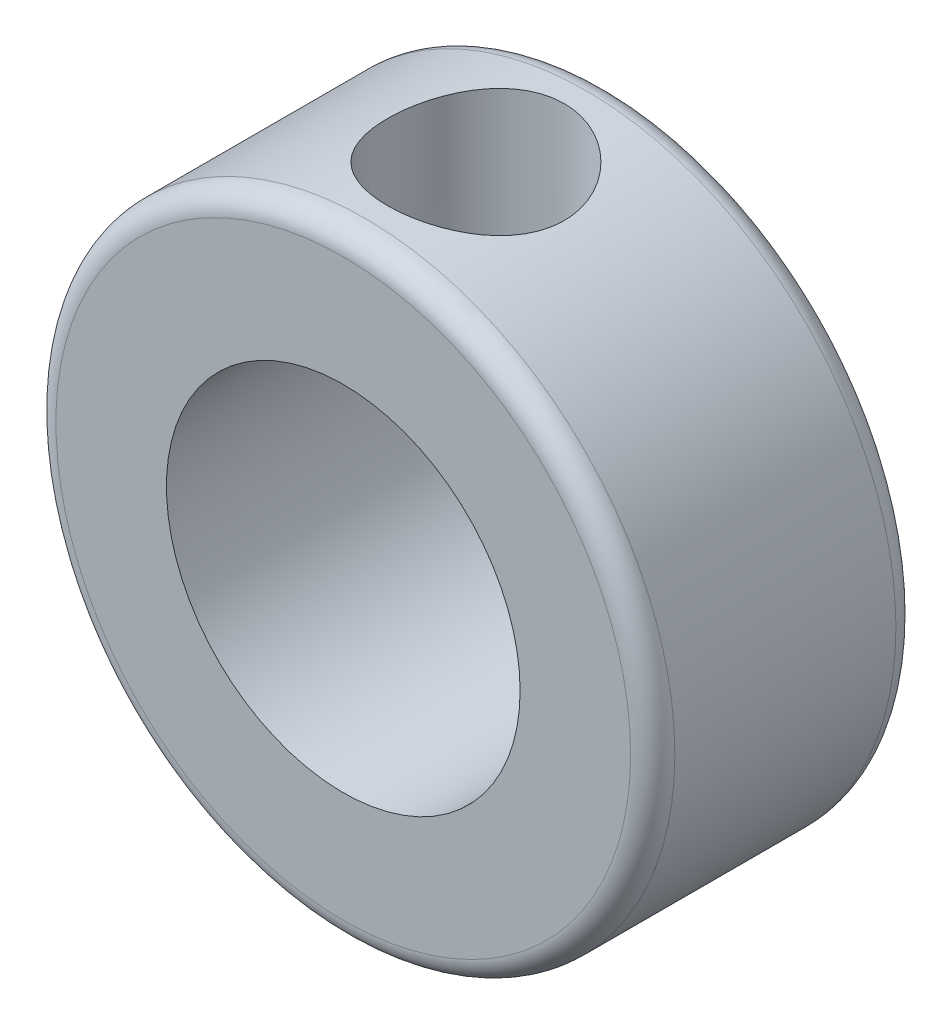
from build123d import *

# Parameters (mm, degrees)
SKETCH1_R           = 14
SKETCH1_R_2         = 8
BOSS_EXTRUDE1_DEPTH = 6
FILLET1_R           = 1
SKETCH2_R           = 4
CUT_EXTRUDE1_DEPTH  = 20


with BuildPart() as part:
    # Sketch1 → Boss-Extrude1 (new, symmetric)
    with BuildSketch(Plane.XY):
        Circle(SKETCH1_R)
        Circle(SKETCH1_R_2, mode=Mode.SUBTRACT)
    extrude(amount=BOSS_EXTRUDE1_DEPTH, both=True)

    # Fillet1
    fillet1_edges = [part.edges().sort_by_distance(p)[0] for p in [
        (-14, 0, -6),
        (-14, 0, 6),
    ]]
    fillet(fillet1_edges, radius=FILLET1_R)

    # Sketch2 → Cut-Extrude1 (cut)
    with BuildSketch(Plane(origin=(0, 0, 0), x_dir=(1, 0, 0), z_dir=(0, 1, 0))):
        with Locations(Location((0, 0, 0), (0, 0, 90))):
            Circle(SKETCH2_R)
    extrude(amount=CUT_EXTRUDE1_DEPTH, mode=Mode.SUBTRACT)


solid = part.part
